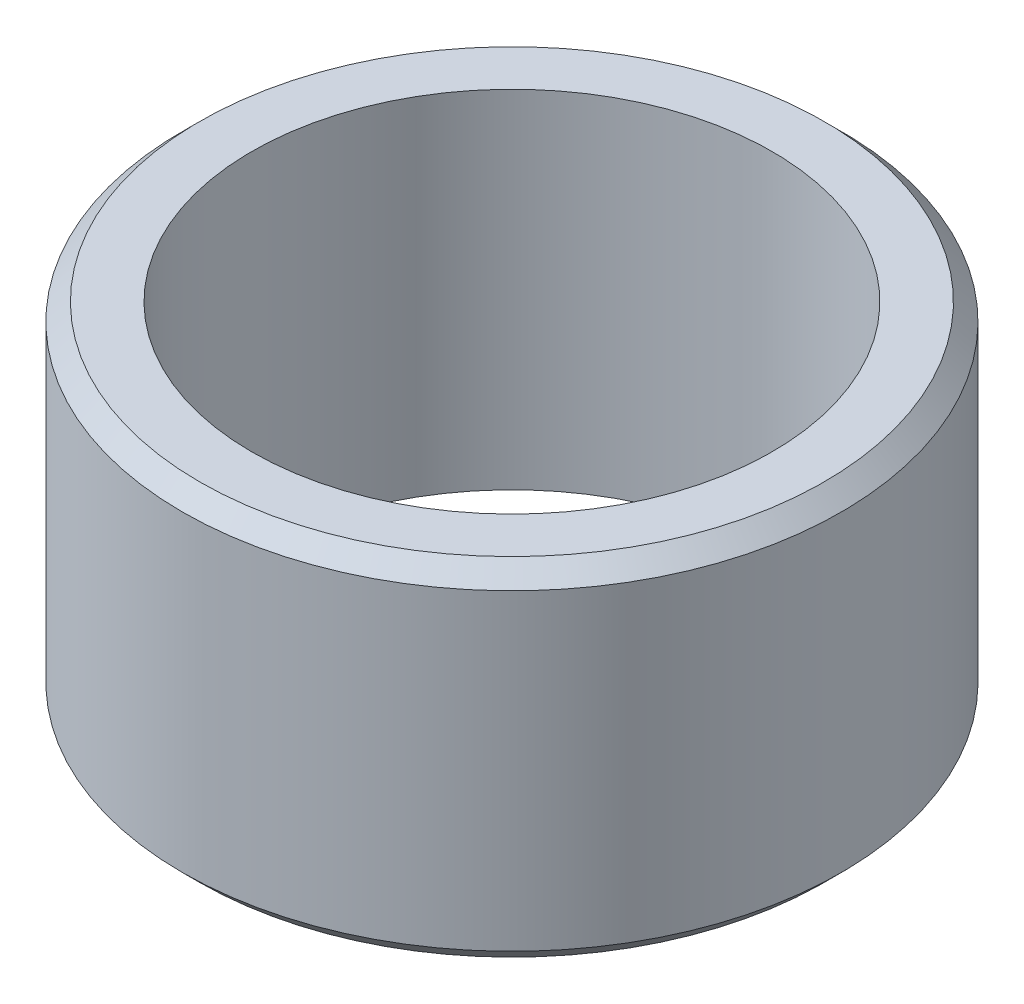
SolidWorks part; units mm, degrees
material "Q235"
ref_plane "Front Plane" through (0, 0, 0) normal (0, 0, 1) x (1, 0, 0)
ref_plane "Top Plane" through (0, 0, 0) normal (0, 1, 0) x (1, 0, 0)
ref_plane "Right Plane" through (0, 0, 0) normal (1, 0, 0) x (0, 0, -1)
sketch "Sketch1" plane through (0, 0, 0) normal (0, 1, 0) x (1, 0, 0)
  circle A0 centre (0, 0) radius 15
  circle A1 centre (0, 0) radius 19
  dimension "D1" = 30
  dimension "D2" = 38
extrude "Boss-Extrude1" add sketch "Sketch1" along normal blind 20
chamfer "Chamfer1" distance 1 angle 45 2 edges at (0, 0, 19) (0, 20, 19)
